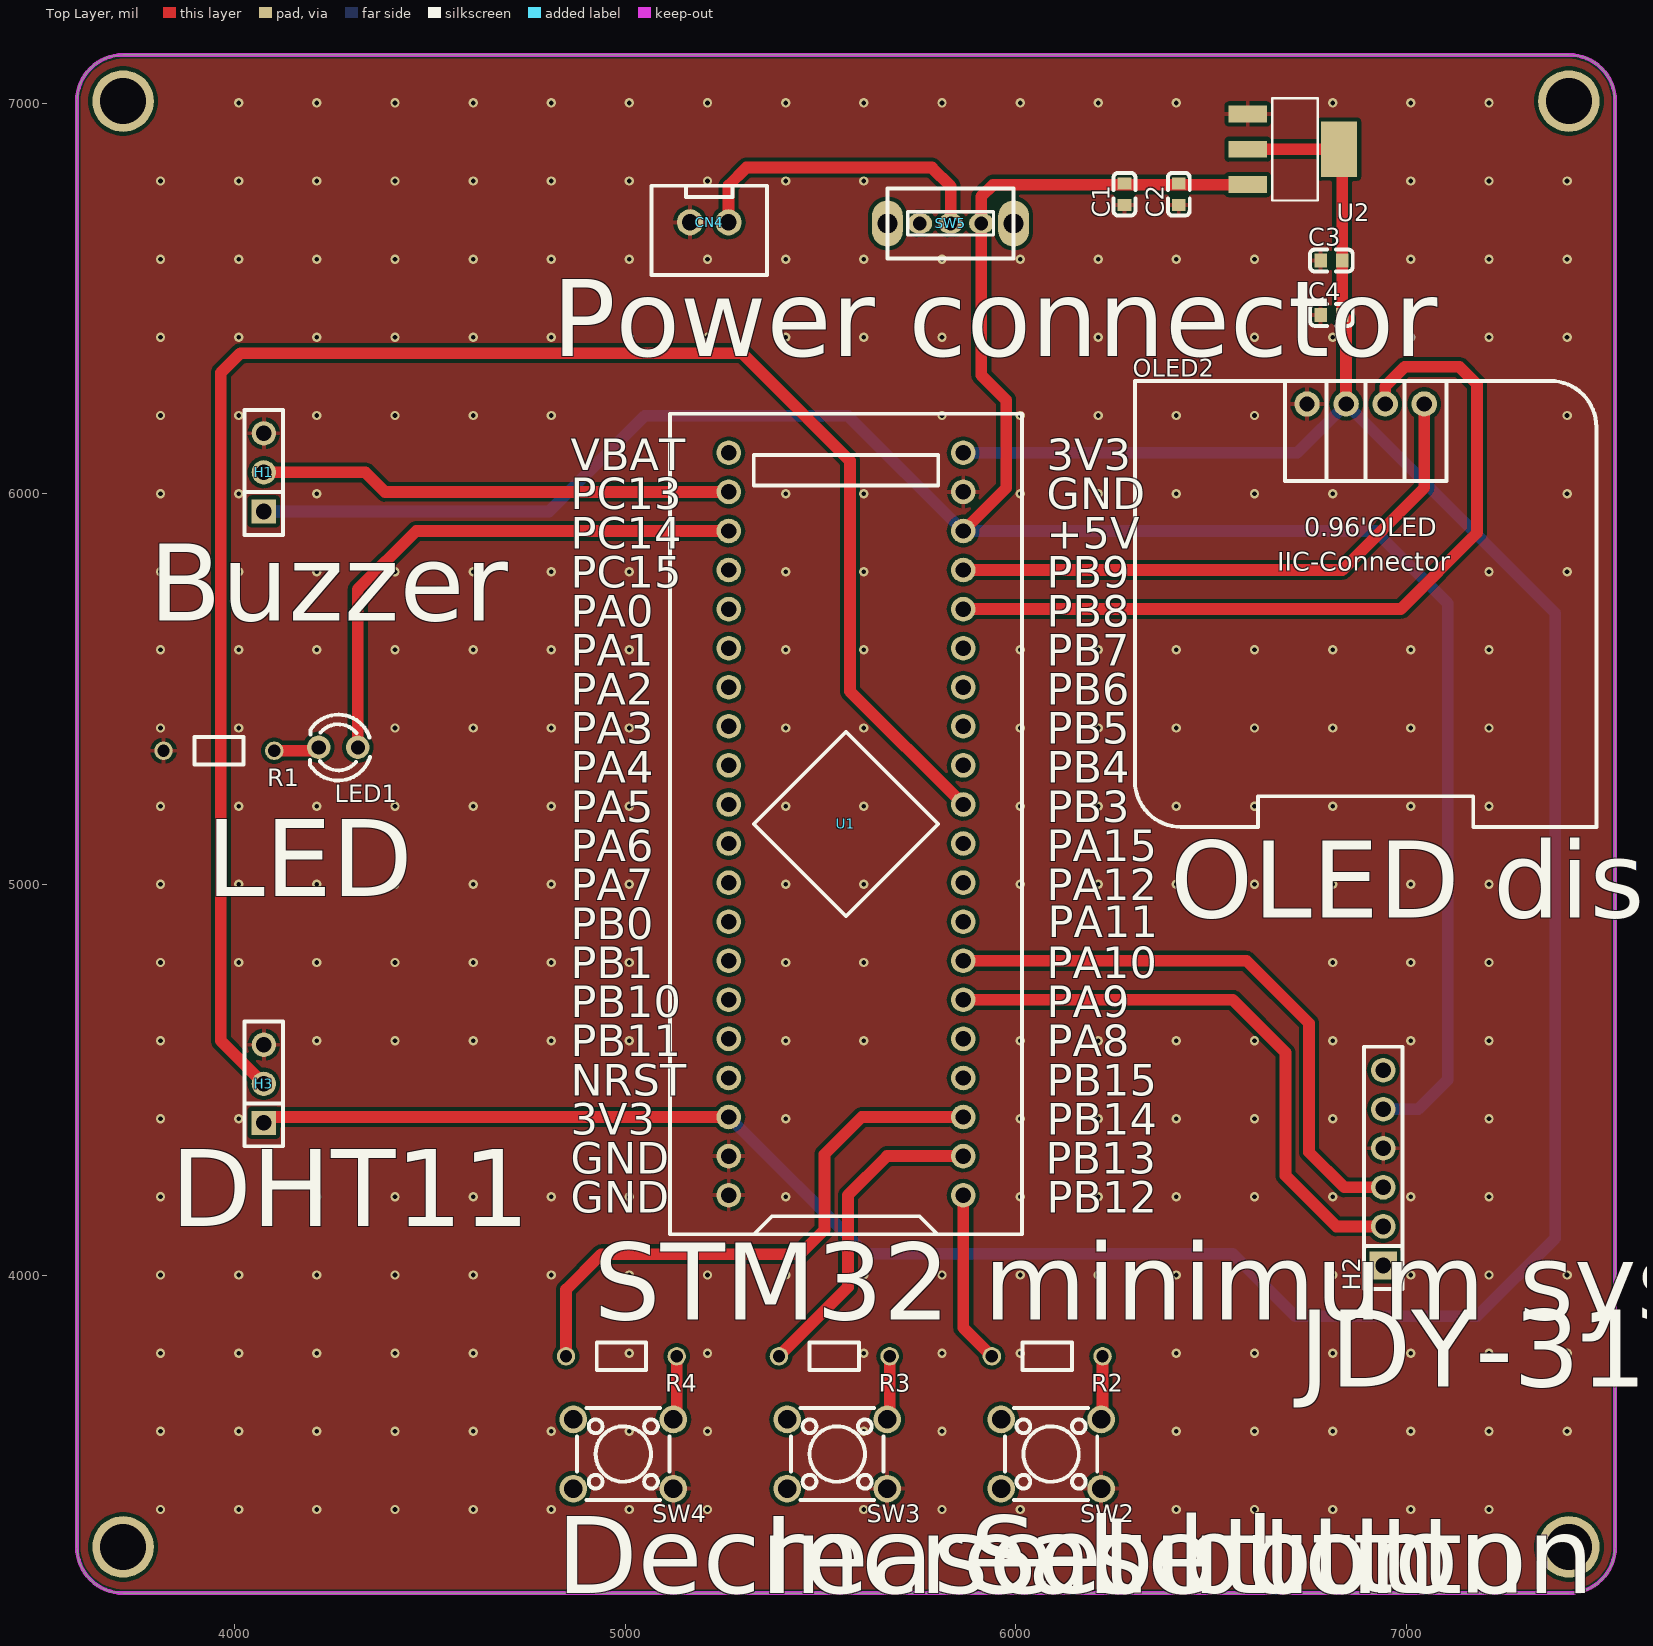
[diagram p0: Top Layer view]
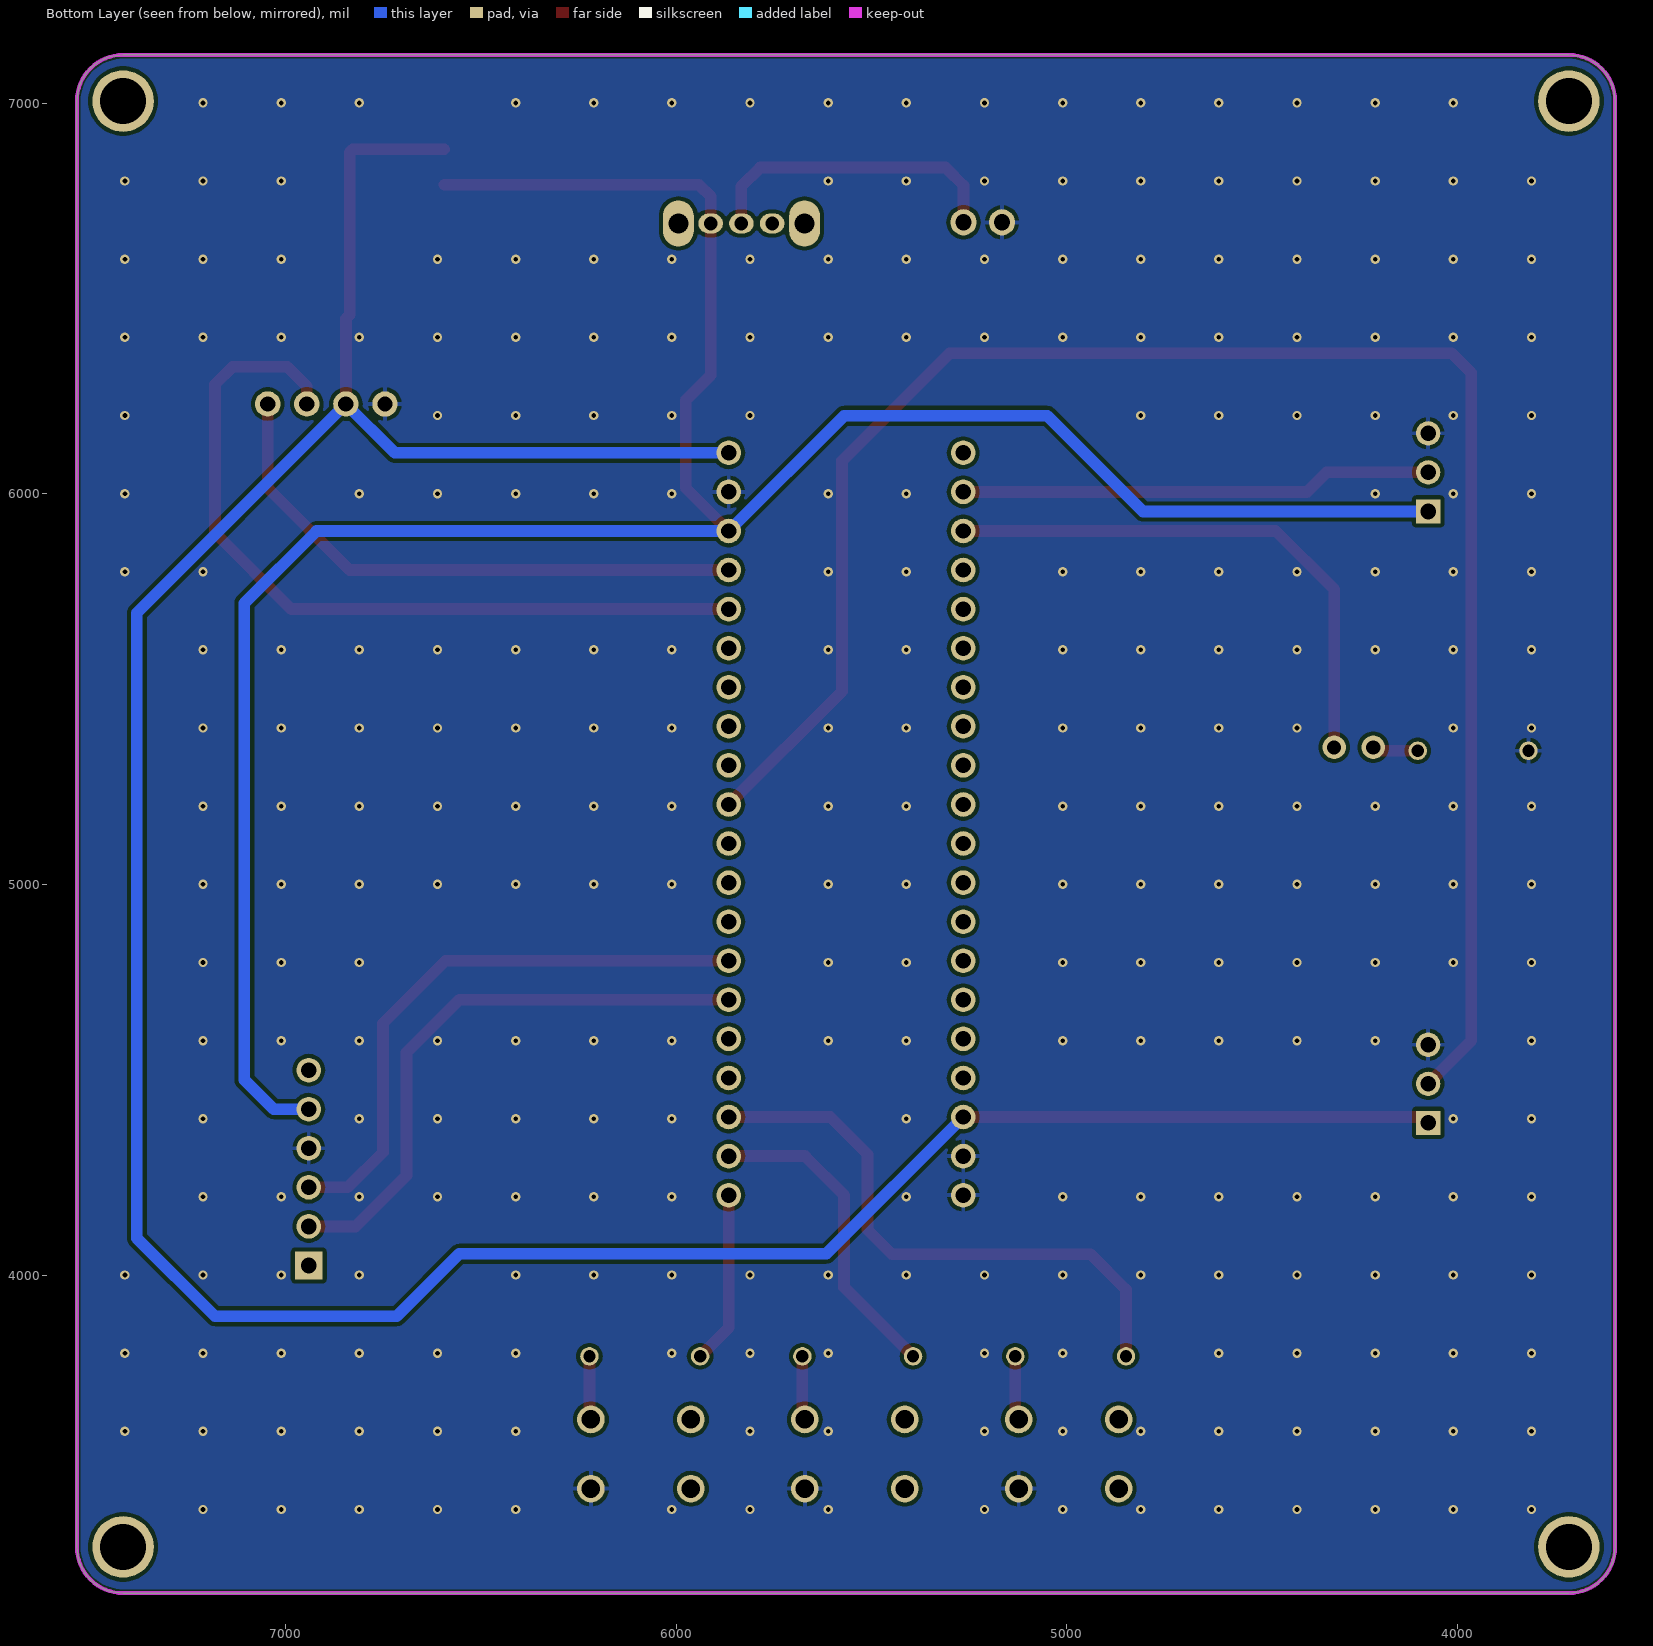
[diagram p1: Bottom Layer view, seen from below]
# Altium PCB MISC51821.pcbdoc
Units mil, origin at the board's own origin, x right, y up, seen from the top; angles counter-clockwise.
Board outline 3937.01 x 3937.01 mil, 2 copper layers (Top Layer, Bottom Layer), stack 62.206 mil thick; 20 components, 42 nets, 101 pads, 280 vias.

## Layer stack, top to bottom
Top Solder Mask Layer: solder mask 0.394, Dk 3.3
Top Layer: signal copper 1.379
Dielectric1: surface 59.449, FR4, Dk 4.5
Bottom Layer: signal copper 1.378
Bottom Solder Mask Layer: solder mask 0.394, Dk 3.3

## Board outline
3714.61,7123.5 ccw(c3714.61,7005.39) 3596.5,7005.39 3596.5,3304.61 ccw(c3714.61,3304.61) 3714.61,3186.5 7415.39,3186.5 ccw(c7415.39,3304.61) 7533.5,3304.61 7533.5,7005.39 ccw(c7415.39,7005.39) 7415.39,7123.5 3714.61,7123.5

## Design rules (kind name [scope] priority, off if disabled: settings)
BoardOutlineClearance copperThickness2oz_1 [All] p2 off: genericclearance=7.99 ignorepadtopadclearanceinfootprint=FALSE except(0: Arc-SplitContinuation Track-SplitContinuation SMDPad-SplitContinuation THPad-SplitContinuation Via-SplitContinuation Fill-SplitContinuation Region-SplitContinuation Poly-SplitContinuation Text-SplitContinuation Hole-SplitContinuation; 5.98: Arc-CutoutEdge Track-CutoutEdge SMDPad-CutoutEdge THPad-CutoutEdge Via-CutoutEdge Text-CutoutEdge; 6.9: Hole-OutlineEdge Hole-CutoutEdge; 10: Poly-OutlineEdge Poly-CutoutEdge; 11.81: Arc-OutlineEdge Track-OutlineEdge SMDPad-OutlineEdge THPad-OutlineEdge Via-OutlineEdge Fill-OutlineEdge Region-OutlineEdge Text-OutlineEdge Fill-CutoutEdge Region-CutoutEdge)
BoardOutlineClearance Plane_innerPlane_1 [All] p4 off: genericclearance=4.02 ignorepadtopadclearanceinfootprint=FALSE except(0: Arc-SplitContinuation Track-SplitContinuation SMDPad-SplitContinuation THPad-SplitContinuation Via-SplitContinuation Fill-SplitContinuation Region-SplitContinuation Poly-SplitContinuation Text-SplitContinuation Hole-SplitContinuation; 5.98: Arc-CutoutEdge Track-CutoutEdge SMDPad-CutoutEdge THPad-CutoutEdge Via-CutoutEdge Text-CutoutEdge; 6.9: Hole-OutlineEdge Hole-CutoutEdge; 10: Poly-OutlineEdge Poly-CutoutEdge; 11.81: Arc-OutlineEdge Track-OutlineEdge SMDPad-OutlineEdge THPad-OutlineEdge Via-OutlineEdge Fill-OutlineEdge Region-OutlineEdge Text-OutlineEdge Fill-CutoutEdge Region-CutoutEdge)
BoardOutlineClearance Copper_copperRegion_1 [All] p6 off: genericclearance=4.02 ignorepadtopadclearanceinfootprint=FALSE except(0: Arc-SplitContinuation Track-SplitContinuation SMDPad-SplitContinuation THPad-SplitContinuation Via-SplitContinuation Fill-SplitContinuation Region-SplitContinuation Poly-SplitContinuation Text-SplitContinuation Hole-SplitContinuation; 5.98: Arc-CutoutEdge Track-CutoutEdge SMDPad-CutoutEdge THPad-CutoutEdge Via-CutoutEdge Text-CutoutEdge; 6.9: Hole-OutlineEdge Hole-CutoutEdge; 10: Poly-OutlineEdge Poly-CutoutEdge; 11.81: Arc-OutlineEdge Track-OutlineEdge SMDPad-OutlineEdge THPad-OutlineEdge Via-OutlineEdge Fill-OutlineEdge Region-OutlineEdge Text-OutlineEdge Fill-CutoutEdge Region-CutoutEdge)
BoardOutlineClearance Copper_copperRegion_copperThickness1oz_1 [All] p8 off: genericclearance=4.02 ignorepadtopadclearanceinfootprint=FALSE except(0: Arc-SplitContinuation Track-SplitContinuation SMDPad-SplitContinuation THPad-SplitContinuation Via-SplitContinuation Fill-SplitContinuation Region-SplitContinuation Poly-SplitContinuation Text-SplitContinuation Hole-SplitContinuation; 5.98: Arc-CutoutEdge Track-CutoutEdge SMDPad-CutoutEdge THPad-CutoutEdge Via-CutoutEdge Text-CutoutEdge; 6.9: Hole-OutlineEdge Hole-CutoutEdge; 10: Poly-OutlineEdge Poly-CutoutEdge; 11.81: Arc-OutlineEdge Track-OutlineEdge SMDPad-OutlineEdge THPad-OutlineEdge Via-OutlineEdge Fill-OutlineEdge Region-OutlineEdge Text-OutlineEdge Fill-CutoutEdge Region-CutoutEdge)
BoardOutlineClearance Copper_copperRegion_Copper_copperRegion_1 [All] p10 off: genericclearance=4.02 ignorepadtopadclearanceinfootprint=FALSE except(0: Arc-SplitContinuation Track-SplitContinuation SMDPad-SplitContinuation THPad-SplitContinuation Via-SplitContinuation Fill-SplitContinuation Region-SplitContinuation Poly-SplitContinuation Text-SplitContinuation Hole-SplitContinuation; 5.98: Arc-CutoutEdge Track-CutoutEdge SMDPad-CutoutEdge THPad-CutoutEdge Via-CutoutEdge Text-CutoutEdge; 6.9: Hole-OutlineEdge Hole-CutoutEdge; 10: Poly-OutlineEdge Poly-CutoutEdge; 11.81: Arc-OutlineEdge Track-OutlineEdge SMDPad-OutlineEdge THPad-OutlineEdge Via-OutlineEdge Fill-OutlineEdge Region-OutlineEdge Text-OutlineEdge Fill-CutoutEdge Region-CutoutEdge)
BoardOutlineClearance copperThickness1oz_1 [All] p12: genericclearance=4.02 ignorepadtopadclearanceinfootprint=FALSE except(0: Arc-SplitContinuation Track-SplitContinuation SMDPad-SplitContinuation THPad-SplitContinuation Via-SplitContinuation Fill-SplitContinuation Region-SplitContinuation Poly-SplitContinuation Text-SplitContinuation Hole-SplitContinuation; 5.98: Arc-CutoutEdge Track-CutoutEdge SMDPad-CutoutEdge THPad-CutoutEdge Via-CutoutEdge Text-CutoutEdge; 6.9: Hole-OutlineEdge Hole-CutoutEdge; 10: Poly-OutlineEdge Poly-CutoutEdge; 11.81: Arc-OutlineEdge Track-OutlineEdge SMDPad-OutlineEdge THPad-OutlineEdge Via-OutlineEdge Fill-OutlineEdge Region-OutlineEdge Text-OutlineEdge Fill-CutoutEdge Region-CutoutEdge)
Clearance copperThickness2oz [All] p1 off: gap=7.99 ignorepadtopadclearanceinfootprint=FALSE except(5.98: SMDPad-Track SMDPad-SMDPad THPad-Track SMDPad-THPad THPad-THPad Track-Via SMDPad-Via THPad-Via Via-Via Fill-SMDPad Region-SMDPad Fill-THPad Region-THPad Fill-Via Region-Via Fill-Fill Fill-Region Region-Region Arc-Track Arc-SMDPad Arc-THPad Arc-Via Fill-Arc Region-Arc Arc-Arc Text-Track SMDPad-Text Text-THPad Text-Via Fill-Text Region-Text Arc-Text Text-Text; 6.9: Hole-Track Hole-SMDPad Hole-THPad Hole-Via Fill-Hole Region-Hole Hole-Arc Hole-Text; 10: Poly-Track Poly-SMDPad Poly-THPad Poly-Via Poly-Fill Poly-Region Poly-Poly Poly-Arc Poly-Text Poly-Hole; 11.81: Fill-Track Region-Track)
Clearance Plane_innerPlane [All] p3 off: gap=4.02 ignorepadtopadclearanceinfootprint=FALSE except(5.98: SMDPad-Track SMDPad-SMDPad THPad-Track SMDPad-THPad THPad-THPad Track-Via SMDPad-Via THPad-Via Via-Via Fill-SMDPad Region-SMDPad Fill-THPad Region-THPad Fill-Via Region-Via Fill-Fill Fill-Region Region-Region Arc-Track Arc-SMDPad Arc-THPad Arc-Via Fill-Arc Region-Arc Arc-Arc Text-Track SMDPad-Text Text-THPad Text-Via Fill-Text Region-Text Arc-Text Text-Text; 6.9: Hole-Track Hole-SMDPad Hole-THPad Hole-Via Fill-Hole Region-Hole Hole-Arc Hole-Text; 10: Poly-Track Poly-SMDPad Poly-THPad Poly-Via Poly-Fill Poly-Region Poly-Poly Poly-Arc Poly-Text Poly-Hole; 11.81: Fill-Track Region-Track)
Clearance Copper_copperRegion [All] p5 off: gap=4.02 ignorepadtopadclearanceinfootprint=FALSE except(5.98: SMDPad-Track SMDPad-SMDPad THPad-Track SMDPad-THPad THPad-THPad Track-Via SMDPad-Via THPad-Via Via-Via Fill-SMDPad Region-SMDPad Fill-THPad Region-THPad Fill-Via Region-Via Fill-Fill Fill-Region Region-Region Arc-Track Arc-SMDPad Arc-THPad Arc-Via Fill-Arc Region-Arc Arc-Arc Text-Track SMDPad-Text Text-THPad Text-Via Fill-Text Region-Text Arc-Text Text-Text; 6.9: Hole-Track Hole-SMDPad Hole-THPad Hole-Via Fill-Hole Region-Hole Hole-Arc Hole-Text; 10: Poly-Track Poly-SMDPad Poly-THPad Poly-Via Poly-Fill Poly-Region Poly-Poly Poly-Arc Poly-Text Poly-Hole; 11.81: Fill-Track Region-Track)
Clearance Copper_copperRegion_copperThickness1oz [All] p7 off: gap=4.02 ignorepadtopadclearanceinfootprint=FALSE except(5.98: SMDPad-Track SMDPad-SMDPad THPad-Track SMDPad-THPad THPad-THPad Track-Via SMDPad-Via THPad-Via Via-Via Fill-SMDPad Region-SMDPad Fill-THPad Region-THPad Fill-Via Region-Via Fill-Fill Fill-Region Region-Region Arc-Track Arc-SMDPad Arc-THPad Arc-Via Fill-Arc Region-Arc Arc-Arc Text-Track SMDPad-Text Text-THPad Text-Via Fill-Text Region-Text Arc-Text Text-Text; 6.9: Hole-Track Hole-SMDPad Hole-THPad Hole-Via Fill-Hole Region-Hole Hole-Arc Hole-Text; 10: Poly-Track Poly-SMDPad Poly-THPad Poly-Via Poly-Fill Poly-Region Poly-Poly Poly-Arc Poly-Text Poly-Hole; 11.81: Fill-Track Region-Track)
Clearance Copper_copperRegion_Copper_copperRegion [All] p9 off: gap=4.02 ignorepadtopadclearanceinfootprint=FALSE except(5.98: SMDPad-Track SMDPad-SMDPad THPad-Track SMDPad-THPad THPad-THPad Track-Via SMDPad-Via THPad-Via Via-Via Fill-SMDPad Region-SMDPad Fill-THPad Region-THPad Fill-Via Region-Via Fill-Fill Fill-Region Region-Region Arc-Track Arc-SMDPad Arc-THPad Arc-Via Fill-Arc Region-Arc Arc-Arc Text-Track SMDPad-Text Text-THPad Text-Via Fill-Text Region-Text Arc-Text Text-Text; 6.9: Hole-Track Hole-SMDPad Hole-THPad Hole-Via Fill-Hole Region-Hole Hole-Arc Hole-Text; 10: Poly-Track Poly-SMDPad Poly-THPad Poly-Via Poly-Fill Poly-Region Poly-Poly Poly-Arc Poly-Text Poly-Hole; 11.81: Fill-Track Region-Track)
Clearance copperThickness1oz [All] p11: gap=4.02 ignorepadtopadclearanceinfootprint=FALSE except(5.98: SMDPad-Track SMDPad-SMDPad THPad-Track SMDPad-THPad THPad-THPad Track-Via SMDPad-Via THPad-Via Via-Via Fill-SMDPad Region-SMDPad Fill-THPad Region-THPad Fill-Via Region-Via Fill-Fill Fill-Region Region-Region Arc-Track Arc-SMDPad Arc-THPad Arc-Via Fill-Arc Region-Arc Arc-Arc Text-Track SMDPad-Text Text-THPad Text-Via Fill-Text Region-Text Arc-Text Text-Text; 6.9: Hole-Track Hole-SMDPad Hole-THPad Hole-Via Fill-Hole Region-Hole Hole-Arc Hole-Text; 10: Poly-Track Poly-SMDPad Poly-THPad Poly-Via Poly-Fill Poly-Region Poly-Poly Poly-Arc Poly-Text Poly-Hole; 11.81: Fill-Track Region-Track)
DiffPairsRouting differentialPair [All] p1: maxlimit=6 minlimit=6 mostfreqgap=6 toplayer_minwidth=5 toplayer_prefwidth=10 toplayer_maxwidth=100 toplayer_mingap=6 toplayer_prefgap=6 toplayer_maxgap=6 bottomlayer_minwidth=5 bottomlayer_prefwidth=10 bottomlayer_maxwidth=100 bottomlayer_mingap=6 bottomlayer_prefgap=6 bottomlayer_maxgap=6 maxuncoupledlength=10
HoleToHoleClearance otherClearance [All] p1: gap=11.81 allowstackedmicrovias=TRUE
Length netLength [All] p1: minlimit=0 maxlimit=0
PasteMaskExpansion pasteMaskExpansion [All] p1: expansion=0
PlaneConnect innerPlane [All] p1: planeconnectstyle=Relief reliefexpansion=20 reliefentries=4 reliefconductorwidth=10 reliefairgap=10
PolygonConnect copperRegion_copperThickness1oz [All] p1 off: connectstyle=Relief reliefconductorwidth=10 reliefentries=4 polygonreliefangle="90 Angle" airgapwidth=10 via.connectstyle=Relief via.reliefconductorwidth=10 via.reliefentries=4 via.polygonreliefangle="90 Angle" via.airgapwidth=10
PolygonConnect copperRegion_Copper_copperRegion [All] p2 off: connectstyle=Relief reliefconductorwidth=10 reliefentries=4 polygonreliefangle="90 Angle" airgapwidth=10 via.connectstyle=Relief via.reliefconductorwidth=10 via.reliefentries=4 via.polygonreliefangle="90 Angle" via.airgapwidth=10
PolygonConnect copperRegion [All] p3: connectstyle=Relief reliefconductorwidth=10 reliefentries=4 polygonreliefangle="90 Angle" airgapwidth=10 via.connectstyle=Relief via.reliefconductorwidth=10 via.reliefentries=4 via.polygonreliefangle="90 Angle" via.airgapwidth=10
RoutingVias viaSize [All] p1: holewidth=12.01 width=24.02 viastyle="Through Hole" minholewidth=11.81 minwidth=19.68 maxholewidth=248.03 maxwidth=393.7
SolderMaskExpansion solderMaskExpansion [IsVia] p1: expansion=-1000 istentingtop=TRUE
SolderMaskExpansion solderMaskExpansion [All] p2: expansion=2 istentingtop=FALSE
Width copperThickness2oz_2 [All] p1 off: maxlimit=100 minlimit=8 preferedwidth=10
Width copperThickness1oz_2 [All] p2: maxlimit=100 minlimit=5 preferedwidth=10

## Components (designator, comment, footprint, x,y, rotation, side; value= is the part's Value field where it differs from the comment)
C1 "100nF" C0603 6277.64,6766.94 r90 top
C2 "10uF" C0603 6416.77,6766.94 r90 top
C3 "100nF" C0603 6807.38,6597.11 r0 top
C4 "10uF" C0603 6807.38,6457.98 r0 top
CN4 "XH2.54*2P_Through-hole" CONN-TH_2P-P2.50-XH2.54-2P 5215,6695 r0 top
H1 "" HDR-TH_3P-P2.54-V-F 4075,6055 r90 top
H2 "" HDR-TH_6P-P2.54-V-F 6940,4275 r90 top
H3 "" HDR-TH_3P-P2.54-V-F 4075,4490 r90 top
LED1 "" LED_TH-3mm 4265.47,5351.27 r180 top
OLED2 "" 0.96OLED_4P 6895,6230 r0 top
R1 "100" Res_1/8W 3960,5345 r180 top
R2 "200Ω" Res_1/8W 6080,3795 r180 top
R3 "200Ω" Res_1/8W 5535,3795 r180 top
R4 "200Ω" Res_1/8W 4990,3795 r180 top
SW2 "" SW-TH_4P-L6.0-W6.0-P4.50-LS6.5 6090,3542.47 r180 top
SW3 "" SW-TH_4P-L6.0-W6.0-P4.50-LS6.5 5542.5,3542.47 r180 top
SW4 "" SW-TH_4P-L6.0-W6.0-P4.50-LS6.5 4995,3542.47 r180 top
SW5 "" 拨动开关 5837.9,6692.05 r180 top
U1 "STM32F103C8T6-Card" CONN-TH_L53.3-W22.9_STM32F103C8T6-CARD 5565,5155 r90 top
U2 "AMS1117-3.3" SOT-223-3_L6.5-W3.4-P2.30-LS7.0-BR 6710.23,6881.95 r180 top

## Footprints (in the part's own frame and the unit in brackets; to place one, negate y for a bottom-side part, rotate by r counter-clockwise, add the part's x,y. Pads: shape width x height; smd on the part's side, far side on the other; paste and mask are expansions set on the pad)
0.96OLED_4P [mm]
  round 1.65 hole 1 copper offset 0,0: 1(-3.81,-0.001) 2(-1.27,0.002) 3(1.27,0.002) 4(3.81,0.002)
  silkscreen extent -15,-27.5 15,1.5
C0603 [mm]
  rect 0.8x0.9 smd: 1(-0.7,0) 2(0.7,0)
  silkscreen extent -1.39,-0.71 1.39,0.71
CONN-TH_2P-P2.50-XH2.54-2P [mm]
  round 1.7 hole 1.05 paste+0 mask+0.05: 1(1.25,0) 2(-1.25,0)
  silkscreen extent -3.75,-3.42 3.75,2.37
CONN-TH_L53.3-W22.9_STM32F103C8T6-CARD [mm]
  round 1.6 hole 1: 1(-24.13,-7.62) 2(-21.59,-7.62) 3(-19.05,-7.62) 4(-16.51,-7.62) 5(-13.97,-7.62) 6(-11.43,-7.62) 7(-8.89,-7.62) 8(-6.35,-7.62) 9(-3.81,-7.62) 10(-1.27,-7.62) 11(1.27,-7.62) 12(3.81,-7.62) 13(6.35,-7.62) 14(8.89,-7.62) 15(11.43,-7.62) 16(13.97,-7.62) 17(16.51,-7.62) 18(19.05,-7.62) 19(21.59,-7.62) 20(24.13,-7.62) 21(24.13,7.62) 22(21.59,7.62) 23(19.05,7.62) 24(16.51,7.62) 25(13.97,7.62) 26(11.43,7.62) 27(8.89,7.62) 28(6.35,7.62) 29(3.81,7.62) 30(1.27,7.62) 31(-1.27,7.62) 32(-3.81,7.62) 33(-6.35,7.62) 34(-8.89,7.62) 35(-11.43,7.62) 36(-13.97,7.62) 37(-16.51,7.62) 38(-19.05,7.62) 39(-21.59,7.62) 40(-24.13,7.62)
  silkscreen extent -26.67,-11.43 26.67,11.43
HDR-TH_3P-P2.54-V-F [mil]
  rect 62x62 hole 40.16: 1(-100,0)
  round 62 hole 40.16: 2(0,0) 3(100,0)
  silkscreen extent -160,-49 160,49
HDR-TH_6P-P2.54-V-F [mm]
  rect 1.8x1.8 hole 1.02: 1(-6.35,0)
  round 1.6 hole 1.02: 2(-3.81,0) 3(-1.27,0) 4(1.27,0) 5(3.81,0) 6(6.35,0)
  silkscreen extent -7.87,-1.25 7.87,1.25
LED_TH-3mm [mil]
  round 60 hole 36 paste+0 mask+2: 1(-50,0) 2(50,0)
  silkscreen extent -81,-84 72,85
Res_1/8W [mil]
  round 47.2 hole 31.5 paste+0 mask+2: 1(-141.7,2.48) 2(141.7,2.48)
  silkscreen extent -63,-33 63,38
SOT-223-3_L6.5-W3.4-P2.30-LS7.0-BR [mm]
  rect 2.5x1.1 smd: 1(2.97,-2.3) 2(2.97,0) 3(2.97,2.3)
  rect 2.34x3.6 smd: 4(-2.97,0)
  silkscreen extent -1.57,-3.33 1.37,3.33
SW-TH_4P-L6.0-W6.0-P4.50-LS6.5 [mm]
  round 1.8 hole 1.2: 1(-3.25,2.25) 2(3.25,2.25) 3(-3.25,-2.25) 4(3.25,-2.25)
  silkscreen extent -3,-3 3,3
拨动开关 [mil]
  oval 63x51.2 hole 35.4 paste+0 mask+2: 1(-73.4,0) 2(5,0) 3(84,0)
  oval 78.7x118.1 hole 51.2 paste+0 mask+2: 4(166.7,0) 5(-156.1,0)
  silkscreen extent -156,-90 167,90

## Free pads (board coordinates)
  round 157.48 hole 118.11: 1(3714.61,7005.39) 1(3714.61,3304.61) 1(7415.39,7005.39) 1(7415.39,3304.61)

## Via types
v1: diameter 24.02, hole 12, Top Layer to Bottom Layer, 280 vias

## Nets (pads, with @x,y where several pads share a name; then routed paths per layer and width w, separated by ;. In a path a pad name is that pad's centre, name@x,y a point inside that pad or via, vN(x,y) a via of type N, cw(c..) or ccw(c..) an arc to the next point about the centre after c; other vN are vias at no path point)
$1N17118: CN4.1 SW5.2 | length 796.8
  Top Layer w30: CN4.1 5264.22,6789.22 5310,6835 5785,6835 5832.9,6787.1 SW5.2
$1N17160: LED1.2 R1.1 | length 117.4
  Top Layer w30: R1.1 4206.72,5342.52 LED1.2
$1N17167: R2.1 SW2.3 | length 163
  Top Layer w30: SW2.3 6221.7,3634.8 R2.1
$1N17169: R3.1 SW3.3 | length 164.1
  Top Layer w30: SW3.3@5670.45,3631.05 5676.7,3637.3 R3.1
$1N17171: R4.1 SW4.3 | length 165.1
  Top Layer w30: SW4.3 5131.7,3639.8 R4.1
+5V: C1.2 C2.2 H1.1 H2.5 SW5.1 U1.18 U2.3 | length 6369.1
  Top Layer w30: U1.18 5975,6015 5975,6240 5911.3,6303.7 SW5.1 5911.3,6761.3 5941.4,6791.4 U2.3
  Bottom Layer w30: H1.1 4805,5955 5050,6200 5570,6200 U1.18 6920,5905 7105,5720 7105,4500 7030,4425 H2.5
GND: C1.1 C2.1 C3.1 C4.1 CN4.2 H1.3 H2.4 H3.3 OLED2.1 R1.2 SW2.1 SW3.1 SW4.1 U1.19 U1.39 U1.40 U2.1
  other v1: 3810.6,3400.6 4010.6,3400.6 4210.6,3400.6 4410.6,3400.6 4610.6,3400.6 4810.6,3400.6 5010.6,3400.6 5210.6,3400.6 5610.6,3400.6 5810.6,3400.6 6010.6,3400.6 6410.6,3400.6 6610.6,3400.6 6810.6,3400.6 7010.6,3400.6 7210.6,3400.6 3810.6,3600.6 4010.6,3600.6 4210.6,3600.6 4410.6,3600.6 4610.6,3600.6 4810.6,3600.6 5010.6,3600.6 5210.6,3600.6 5610.6,3600.6 5810.6,3600.6 6410.6,3600.6 6610.6,3600.6 6810.6,3600.6 7010.6,3600.6 7210.6,3600.6 7410.6,3600.6 3810.6,3800.6 4010.6,3800.6 4210.6,3800.6 4410.6,3800.6 4610.6,3800.6 5010.6,3800.6 5210.6,3800.6 5610.6,3800.6 5810.6,3800.6 6010.6,3800.6 6410.6,3800.6 6610.6,3800.6 6810.6,3800.6 7010.6,3800.6 7210.6,3800.6 7410.6,3800.6 3810.6,4000.6 4010.6,4000.6 4210.6,4000.6 4410.6,4000.6 4610.6,4000.6 4810.6,4000.6 5010.6,4000.6 5210.6,4000.6 5410.6,4000.6 5610.6,4000.6 5810.6,4000.6 6010.6,4000.6 6210.6,4000.6 6410.6,4000.6 6810.6,4000.6 7010.6,4000.6 7210.6,4000.6 7410.6,4000.6 3810.6,4200.6 4010.6,4200.6 4210.6,4200.6 4410.6,4200.6 4610.6,4200.6 4810.6,4200.6 5010.6,4200.6 5410.6,4200.6 6010.6,4200.6 6210.6,4200.6 6410.6,4200.6 6610.6,4200.6 6810.6,4200.6 7010.6,4200.6 7210.6,4200.6 3810.6,4400.6 4010.6,4400.6 5410.6,4400.6 6010.6,4400.6 6210.6,4400.6 6410.6,4400.6 6610.6,4400.6 6810.6,4400.6 7210.6,4400.6 3810.6,4600.6 4210.6,4600.6 4410.6,4600.6 4610.6,4600.6 4810.6,4600.6 5010.6,4600.6 5410.6,4600.6 5610.6,4600.6 6010.6,4600.6 6210.6,4600.6 6410.6,4600.6 6610.6,4600.6 6810.6,4600.6 7010.6,4600.6 7210.6,4600.6 3810.6,4800.6 4010.6,4800.6 4210.6,4800.6 4410.6,4800.6 4610.6,4800.6 4810.6,4800.6 5010.6,4800.6 5410.6,4800.6 5610.6,4800.6 6810.6,4800.6 7010.6,4800.6 7210.6,4800.6 3810.6,5000.6 4010.6,5000.6 4210.6,5000.6 4410.6,5000.6 4610.6,5000.6 4810.6,5000.6 5010.6,5000.6 5410.6,5000.6 5610.6,5000.6 6010.6,5000.6 6210.6,5000.6 6410.6,5000.6 6610.6,5000.6 6810.6,5000.6 7010.6,5000.6 7210.6,5000.6 3810.6,5200.6 4010.6,5200.6 4210.6,5200.6 4410.6,5200.6 4610.6,5200.6 4810.6,5200.6 5010.6,5200.6 5410.6,5200.6 5610.6,5200.6 6010.6,5200.6 6210.6,5200.6 6410.6,5200.6 6610.6,5200.6 6810.6,5200.6 7010.6,5200.6 7210.6,5200.6 3810.6,5400.6 4010.6,5400.6 4410.6,5400.6 4610.6,5400.6 4810.6,5400.6 5010.6,5400.6 5410.6,5400.6 5610.6,5400.6 6010.6,5400.6 6210.6,5400.6 6410.6,5400.6 6610.6,5400.6 6810.6,5400.6 7010.6,5400.6 7210.6,5400.6 3810.6,5600.6 4010.6,5600.6 4210.6,5600.6 4410.6,5600.6 4610.6,5600.6 4810.6,5600.6 5010.6,5600.6 5410.6,5600.6 5610.6,5600.6 6010.6,5600.6 6210.6,5600.6 6410.6,5600.6 6610.6,5600.6 6810.6,5600.6 7010.6,5600.6 7210.6,5600.6 3810.6,5800.6 4010.6,5800.6 4210.6,5800.6 4410.6,5800.6 4610.6,5800.6 4810.6,5800.6 5010.6,5800.6 5410.6,5800.6 5610.6,5800.6 7210.6,5800.6 7410.6,5800.6 3810.6,6000.6 4010.6,6000.6 4210.6,6000.6 5410.6,6000.6 5610.6,6000.6 6010.6,6000.6 6210.6,6000.6 6410.6,6000.6 6610.6,6000.6 6810.6,6000.6 7410.6,6000.6 3810.6,6200.6 4010.6,6200.6 4210.6,6200.6 4410.6,6200.6 4610.6,6200.6 4810.6,6200.6 5810.6,6200.6 6010.6,6200.6 6210.6,6200.6 6410.6,6200.6 6610.6,6200.6 7410.6,6200.6 3810.6,6400.6 4010.6,6400.6 4210.6,6400.6 4410.6,6400.6 4610.6,6400.6 4810.6,6400.6 5010.6,6400.6 5210.6,6400.6 5410.6,6400.6 5610.6,6400.6 5810.6,6400.6 6010.6,6400.6 6210.6,6400.6 6410.6,6400.6 6610.6,6400.6 6810.6,6400.6 7010.6,6400.6 7210.6,6400.6 7410.6,6400.6 3810.6,6600.6 4010.6,6600.6 4210.6,6600.6 4410.6,6600.6 4610.6,6600.6 4810.6,6600.6 5010.6,6600.6 5210.6,6600.6 5410.6,6600.6 5610.6,6600.6 5810.6,6600.6 6010.6,6600.6 6210.6,6600.6 6410.6,6600.6 6610.6,6600.6 7010.6,6600.6 7210.6,6600.6 7410.6,6600.6 3810.6,6800.6 4010.6,6800.6 4210.6,6800.6 4410.6,6800.6 4610.6,6800.6 4810.6,6800.6 5010.6,6800.6 5210.6,6800.6 5410.6,6800.6 5610.6,6800.6 7010.6,6800.6 7210.6,6800.6 7410.6,6800.6 4010.6,7000.6 4210.6,7000.6 4410.6,7000.6 4610.6,7000.6 4810.6,7000.6 5010.6,7000.6 5210.6,7000.6 5410.6,7000.6 5610.6,7000.6 5810.6,7000.6 6010.6,7000.6 6210.6,7000.6 6410.6,7000.6 6810.6,7000.6 7010.6,7000.6 7210.6,7000.6
NRST: U1.37
PA0: U1.25
PA1: U1.26
PA2: U1.27
PA3: U1.28
PA4: U1.29
PA5: U1.30
PA6: U1.31
PA7: U1.32
PA8: U1.5
PA9: H2.2 U1.6 | length 1499.8
  Top Layer w30: U1.6 6555,4705 6690,4570 6690,4255 6820,4125 H2.2
PA10: H2.3 U1.7 | length 1508.6
  Top Layer w30: U1.7 6590,4805 6750,4645 6750,4315 6840,4225 H2.3
PA11: U1.8
PA12: U1.9
PA15: U1.10
PB0: U1.33
PB1: U1.34
PB3: H3.2 U1.11 | length 4610.3
  Top Layer w30: H3.2 3965,4600 3965,6310 4015,6360 5300,6360 5575,6085 5575,5495 U1.11
PB4: U1.12
PB5: U1.13
PB6: U1.14
PB7: U1.15
PB8: OLED2.3 U1.16 | length 2095.1
  Top Layer w30: U1.16 6985,5705 7180,5900 7180,6280 7135,6325 6995,6325 6945,6275 OLED2.3@6945,6230.05
PB9: OLED2.4 U1.17 | length 1482
  Top Layer w30: U1.17 6835,5805 7045,6015 OLED2.4@7045,6230.05
PB10: U1.35
PB11: U1.36
PB12: R2.2 U1.1 | length 442.8
  Top Layer w30: U1.1 5865,3865.82 R2.2
PB13: R3.2 U1.2 | length 822.1
  Top Layer w30: R3.2 5570,3969.22 5570,4205 5670,4305 U1.2
PB14: R4.2 U1.3 | length 1483.8
  Top Layer w30: R4.2 4848.3,3963.3 4938.79,4053.79 5447.34,4053.79 5510,4116.45 5510,4310 5605,4405 U1.3
PB15: U1.4
PC13: H1.2 U1.22 | length 1210.7
  Top Layer w30: H1.2 4335,6055 4385,6005 U1.22
PC14: LED1.1 U1.23 | length 1415.7
  Top Layer w30: LED1.1 4315.47,5755.47 4465,5905 U1.23
PC15: U1.24
VBAT: U1.21
VCC: C3.2 C4.2 H3.1 OLED2.2 U1.20 U1.38 U2.2 U2.4 | length 7886.9
  Top Layer w30: H3.1 4090,4405 U1.38 ; U2.2 U2.4 6834.94,6874.17 C3.2 C4.2 6845,6447.91 OLED2.2@6845,6230.05
  Bottom Layer w30: U1.38 5615,4055 6555,4055 6715,3895 7180,3895 7380,4095 7380,5695.05 6845,6230.05 6719.95,6105 U1.20
pads on no net: H2.1 H2.6 SW2.2 SW2.4 SW3.2 SW3.4 SW4.2 SW4.4 SW5.3 SW5.4 SW5.5

## Polygon pours and split planes (outlines as drawn)
GND on Bottom Layer (solid, remove dead copper, pour order 2): 3525,7245 3525,3080 7700,3080 7700,7245
GND on Top Layer (solid, remove dead copper, pour order 2): 3000,7415 3000,3000 7930,3000 7930,7415

## Keep-outs
Board Outline Layer:
  the board outline again, w10

## Silkscreen, mask and mechanical layers (free items; w line width, h text height)
Top Silkscreen Layer:
  text "Power connector" at 4812.87,6351.57 h196.85
  text "VBAT" at 4860.95,6060 h80
  text "3V3" at 6079.16,6060 h80
  text "PC13" at 4860.95,5960 h80
  text "GND" at 6079.16,5960 h80
  text "PC14" at 4860.95,5860 h80
  text "+5V" at 6079.16,5860 h80
  text "PC15" at 4860.95,5760 h80
  text "PB9" at 6079.16,5760 h80
  text "Buzzer" at 3781.81,5675 h196.85
  text "PA0" at 4860.95,5660 h80
  text "PB8" at 6079.16,5660 h80
  text "PA1" at 4860.95,5560 h80
  text "PB7" at 6079.16,5560 h80
  text "PA2" at 4860.95,5460 h80
  text "PB6" at 6079.16,5460 h80
  text "PA3" at 4860.95,5360 h80
  text "PB5" at 6079.16,5360 h80
  text "PA4" at 4860.95,5260 h80
  text "PB4" at 6079.16,5260 h80
  text "PA5" at 4860.95,5160 h80
  text "PB3" at 6079.16,5160 h80
  text "PA6" at 4860.95,5060 h80
  text "PA15" at 6079.16,5060 h80
  text "LED" at 3927.96,4970 h196.85
  text "PA7" at 4860.95,4960 h80
  text "PA12" at 6079.16,4960 h80
  text "OLED display" at 6395,4915 h196.85
  text "PA11" at 6080.95,4865 h80
  text "PB0" at 4860.95,4860 h80
  text "PB1" at 4860.95,4760 h80
  text "PA10" at 6079.16,4760 h80
  text "PB10" at 4860.95,4660 h80
  text "PA9" at 6079.16,4660 h80
  text "PB11" at 4860.95,4560 h80
  text "PA8" at 6079.16,4560 h80
  text "NRST" at 4860.95,4460 h80
  text "PB15" at 6079.16,4460 h80
  text "3V3" at 4860.95,4360 h80
  text "PB14" at 6079.16,4360 h80
  text "GND" at 4860.95,4260 h80
  text "PB13" at 6075.95,4260 h80
  text "GND" at 4860.95,4160 h80
  text "PB12" at 6079.16,4160 h80
  text "DHT11" at 3836.39,4125 h196.85
  text "STM32 minimum system" at 4919.45,3886.57 h196.85
  text "JDY-31" at 6725,3715 h196.85
  text "Increase button" at 5353.14,3186.57 h196.85
  text "Set button" at 5883.15,3187.47 h196.85
  text "Decrease button" at 4825,3185.68 h196.85